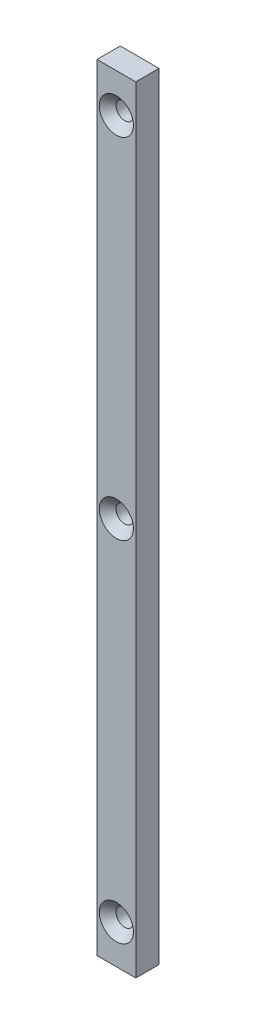
SolidWorks part; units mm, degrees
material "45#"
ref_plane "Front Plane" through (0, 0, 0) normal (0, 0, 1) x (1, 0, 0)
ref_plane "Top Plane" through (0, 0, 0) normal (0, 1, 0) x (1, 0, 0)
ref_plane "Right Plane" through (0, 0, 0) normal (1, 0, 0) x (0, 0, -1)
sketch "Sketch1" plane through (0, 0, 0) normal (0, 0, 1) x (1, 0, 0)
  line L1 (0, 0) -> (20, 0)
  line L2 (0, 0) -> (0, 400)
  line L3 (0, 400) -> (20, 400)
  line L4 (20, 0) -> (20, 400)
  dimension "D1" = 20
  dimension "D2" = 400
extrude "Boss-Extrude1" add sketch "Sketch1" along normal blind 12
hole_wizard "Hole size (by hex socket flat countersunk head screw type)1" positions "Sketch2" profile "Sketch3" countersink size "M8" standard "GB" end condition through all
sketch "Sketch2" plane through (0, 0, 12) normal (0, 0, 1) x (1, 0, 0)
  line L0 (10, 400) -> (10, 380) construction
  line L1 (20, 400) -> (0, 400) construction
  line L3 (0, 0) -> (20, 0) construction
  line L4 (0, 200) -> (10, 200) construction
  line L5 (0, 400) -> (0, 0) construction
  point P0 (10, 380)
  point P2 (10, 200)
  point P11 (10, 20)
  dimension "D1" = 20
  dimension "D3" = 20
sketch "Sketch3" plane through (10, 380, 12) normal (1, 0, 0) x (0, -1, 0)
  line L0 (0, 0) -> (0, 12)
  line L1 (0, 12) -> (4.5, 12)
  line L2 (4.5, 12) -> (4.5, 4.3)
  line L3 (4.5, 4.3) -> (8.8, 0)
  line L5 (8.8, 0) -> (0, 0)
  line L6 (-4.5, 4.3) -> (-8.8, 0) construction
  line L11 (0, -6.35) -> (0, 107.95) construction
  dimension "通孔孔直径" = 9
  dimension "通孔孔深度" = 12
  dimension "近端锥形沉头孔直径" = 17.6
  dimension "近端锥形沉头孔角度" = 90
